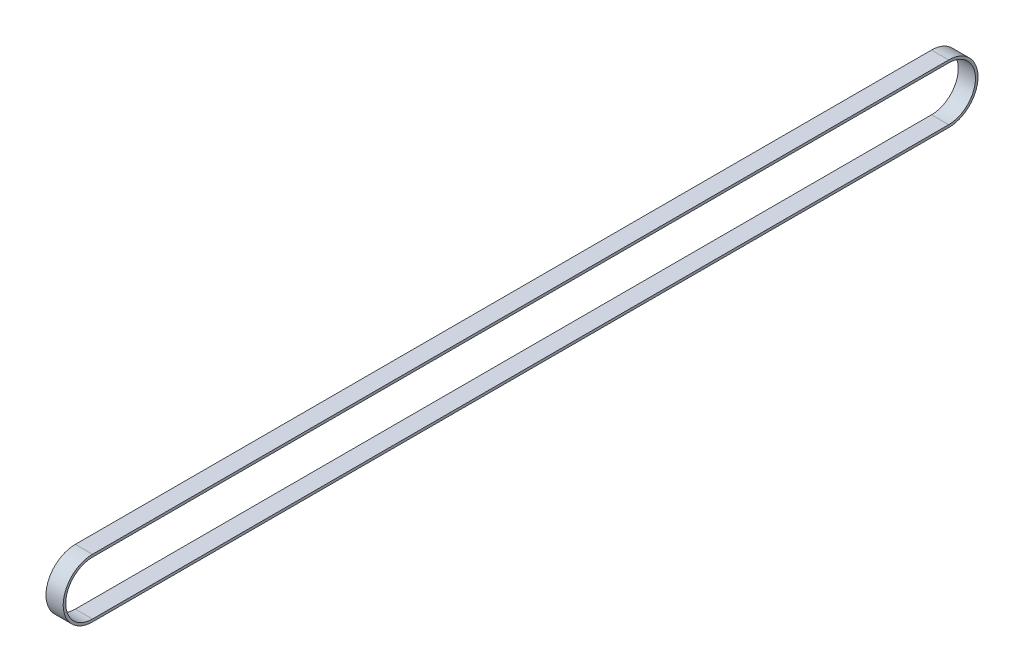
from build123d import *

# Parameters (mm, degrees)
EXTRUDE_1_DEPTH = 15


with BuildPart() as part:
    # 草图2 → 拉伸-薄壁1 (new, symmetric)
    with BuildSketch(Plane(origin=(0, 0, 0), x_dir=(0, 0, -1), z_dir=(1, 0, 0))):
        with BuildLine():
            Line((-1496.41, -51.25), (0, -51.25))
            ThreePointArc((0, -51.25), (51.25, 0), (0, 51.25))
            Line((0, 51.25), (-1496.41, 51.25))
            ThreePointArc((-1496.41, 51.25), (-1547.66, 0), (-1496.41, -51.25))
        make_face()
        with BuildLine():
            Line((-1496.41, -46.75), (0, -46.75))
            ThreePointArc((0, -46.75), (46.75, 0), (0, 46.75))
            Line((0, 46.75), (-1496.41, 46.75))
            ThreePointArc((-1496.41, 46.75), (-1543.16, 0), (-1496.41, -46.75))
        make_face(mode=Mode.SUBTRACT)
    extrude(amount=EXTRUDE_1_DEPTH, both=True)


solid = part.part
